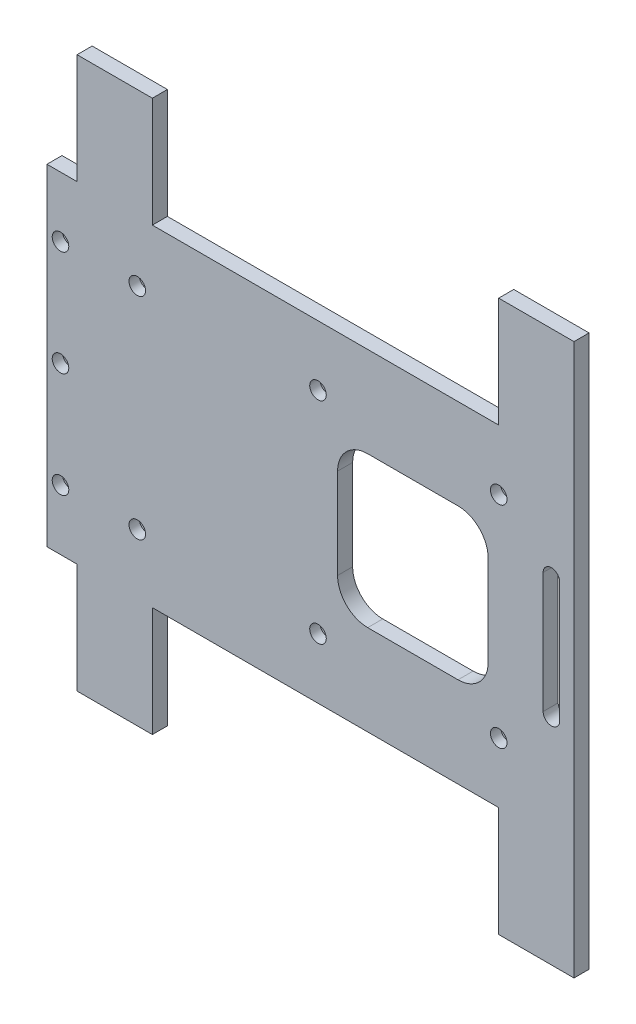
SolidWorks part; units mm, degrees
material "6061 合金"
ref_plane "前视基准面" through (0, 0, 0) normal (0, 0, 1) x (1, 0, 0)
ref_plane "上视基准面" through (0, 0, 0) normal (0, 1, 0) x (1, 0, 0)
ref_plane "右视基准面" through (0, 0, 0) normal (1, 0, 0) x (0, 0, -1)
sketch "草图1" plane through (0, 0, 0) normal (0, 0, 1) x (1, 0, 0)
  line L1 (175, -110) -> (-175, -110)
  line L2 (175, -110) -> (175, 110)
  line L3 (175, 110) -> (-175, 110)
  line L4 (-175, -110) -> (-175, 110)
  line L5 (175, -110) -> (-175, 110) construction
  line L6 (175, 110) -> (-175, -110) construction
  point P0 (0, 0)
  dimension "D1" = 350
  dimension "D2" = 220
extrude "凸台-拉伸1" add sketch "草图1" along normal mid plane 10
sketch "草图2" plane through (0, 0, 5) normal (0, 0, 1) x (1, 0, 0)
  line L0 (-213.5, 40) -> (-213.5, -40) construction
  line L1 (-208, 40) -> (-208, -40)
  line L2 (-219, 40) -> (-219, -40)
  line L3 (160, 40) -> (160, -40) construction
  line L4 (165.5, 40) -> (165.5, -40)
  line L5 (154.5, 40) -> (154.5, -40)
  line L6 (175, -110) -> (175, 110) construction
  arc A0 (-208, 40) -> (-219, 40) centre (-213.5, 40) ccw
  arc A1 (-219, -40) -> (-208, -40) centre (-213.5, -40) ccw
  arc A2 (165.5, 40) -> (154.5, 40) centre (160, 40) ccw
  arc A3 (154.5, -40) -> (165.5, -40) centre (160, -40) ccw
  point P2 (-213.5, 0)
  point P7 (160, 0)
  dimension "D1" = 11
  dimension "D2" = 80
  dimension "D3" = 373.5
  dimension "D4" = 15
extrude "切除-拉伸1" cut sketch "草图2" against normal through all
sketch "草图4" plane through (0, 0, 5) normal (0, 0, 1) x (1, 0, 0)
  line L0 (175, -110) -> (175, 110) construction
  line L1 (160, -95) -> (-213.5, -95)
  line L2 (160, -95) -> (160, 95)
  line L3 (160, 95) -> (-213.5, 95)
  line L4 (-213.5, -95) -> (-213.5, 95)
  line L5 (160, -95) -> (-213.5, 95) construction
  line L6 (160, 95) -> (-213.5, -95) construction
  point P0 (-26.75, 0)
  point P6 (175, 0)
  dimension "D1" = 373.5
  dimension "D2" = 190
  dimension "D3" = 15
sketch "草图6" plane through (0, 0, 5) normal (0, 0, 1) x (1, 0, 0)
  line L1 (98, -50) -> (38, -50)
  line L2 (118, -30) -> (118, 30)
  line L3 (98, 50) -> (38, 50)
  line L4 (18, -30) -> (18, 30)
  line L5 (118, -50) -> (18, 50) construction
  line L6 (118, 50) -> (18, -50) construction
  line L8 (175, -110) -> (175, 110) construction
  arc A0 (98, 50) -> (118, 30) centre (98, 30) cw
  arc A1 (118, -30) -> (98, -50) centre (98, -30) cw
  arc A2 (38, -50) -> (18, -30) centre (38, -30) cw
  arc A3 (18, 30) -> (38, 50) centre (38, 30) cw
  point P0 (68, 0)
  dimension "D3" = 20
  dimension "D1" = 100
  dimension "D2" = 100
  dimension "D4" = 57
extrude "切除-拉伸2" cut sketch "草图6" against normal through all
hole_wizard "打孔尺寸(%根据)内六角圆柱头螺钉的类型1" positions "3D草图2" profile "草图7" counterbore size "M6" standard "GB"
sketch3d "3D草图2"
  line L0 (-175, 110, 5) -> (-175, -110, 5) construction
  line L1 (-175, -110, 5) -> (175, -110, 5) construction
  line L2 (175, 110, 5) -> (-175, 110, 5) construction
  point P0 (-115, 70, 5)
  point P10 (-115, -70, 5)
  point P13 (-166, 70, 5)
  point P15 (-166, -70, 5)
  point P24 (-166, 0, 5)
  point P27 (5, 70, 5)
  point P29 (125, 70, 5)
  point P31 (125, -70, 5)
  point P33 (5, -70, 5)
  dimension "D1" = 9
  dimension "D2" = 9
  dimension "D3" = 40
  dimension "D4" = 40
  dimension "D5" = 40
  dimension "D6" = 60
  dimension "D7" = 60
  dimension "D8" = 40
  dimension "D9" = 9
  dimension "D10" = 110
  dimension "D11" = 40
  dimension "D12" = 40
  dimension "D13" = 120
  dimension "D14" = 120
  dimension "D15" = 40
  dimension "D16" = 40
  dimension "D17" = 120
  dimension "D18" = 120
sketch "草图7" plane through (-115, 70, 5) normal (1, 0, 0) x (0, -1, 0)
  line L0 (0, 0) -> (0, 16.9828)
  line L1 (0, 16.9828) -> (3.3, 15)
  line L2 (3.3, 15) -> (3.3, 6.8)
  line L3 (3.3, 6.8) -> (5.5, 6.8)
  line L4 (5.5, 6.8) -> (5.5, 0)
  line L5 (5.5, 0) -> (0, 0)
  line L10 (0, 16.9828) -> (-3.3, 15) construction
  line L11 (0, -6.35) -> (0, 107.95) construction
  dimension "孔直径" = 6.6
  dimension "孔深度" = 15
  dimension "柱形沉头孔直径" = 11
  dimension "柱形沉头孔深度" = 6.8
  dimension "导头角度" = 118
sketch "草图8" plane through (0, 0, -5) normal (0, 0, -1) x (-1, 0, 0)
  line L1 (-175, 110) -> (-125, 110)
  line L2 (-175, 110) -> (-175, 183)
  line L3 (-175, 183) -> (-125, 183)
  line L4 (-125, 110) -> (-125, 183)
  line L5 (-175, -110) -> (-125, -110)
  line L6 (-175, -110) -> (-175, -183)
  line L7 (-175, -183) -> (-125, -183)
  line L8 (-125, -110) -> (-125, -183)
  dimension "D1" = 73
  dimension "D2" = 50
extrude "凸台-拉伸2" add sketch "草图8" against normal up to surface (10 mm away) up to face at (-109.5, 70, 5)
pattern_linear "阵列(线性)1" count 2 spacing 280 along (-1, 0, 0) of "凸台-拉伸2"
